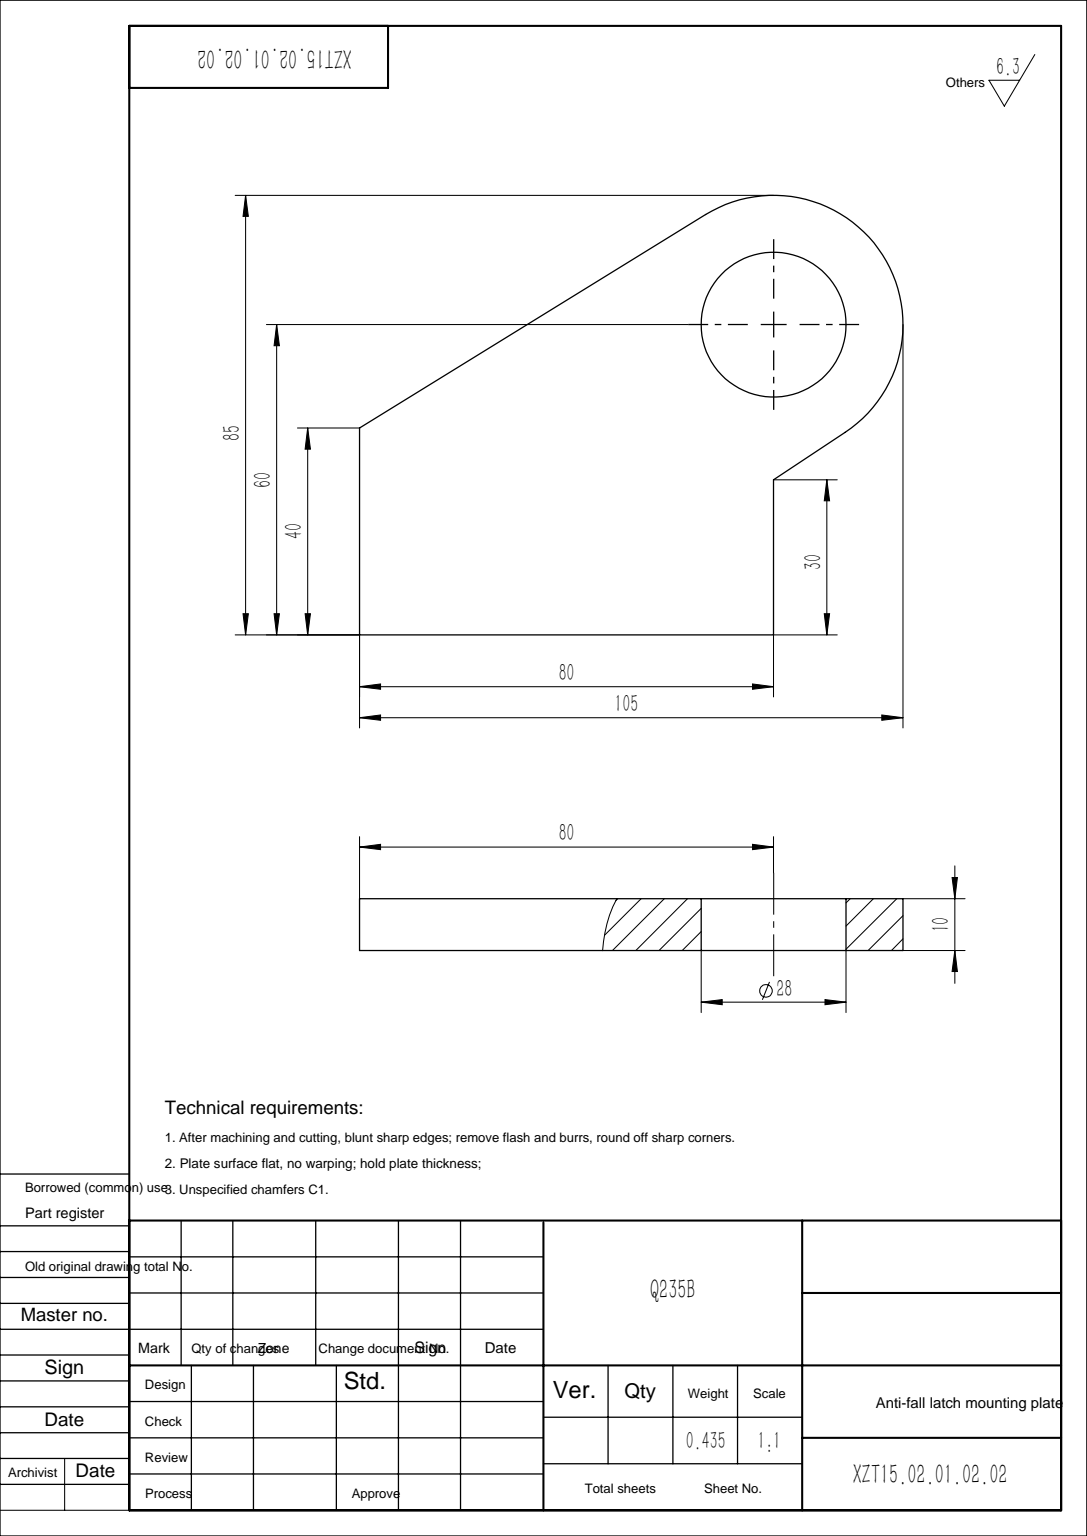
from build123d import *

# Parameters (mm, degrees)
SKETCH1_R           = 14
BOSS_EXTRUDE1_DEPTH = 5


with BuildPart() as part:
    # Sketch1 → Boss-Extrude1 (new, symmetric)
    with BuildSketch(Plane.XY):
        with BuildLine():
            Line((0, 0), (0, 40))
            Line((0, 40), (66.869031748, 81.273873008))
            ThreePointArc((66.869031748, 81.273873008), (101.056415799, 73.476919296), (93.81926996, 39.166666667))
            Line((93.81926996, 39.166666667), (80, 30))
            Line((80, 30), (80, 0))
            Line((80, 0), (0, 0))
        make_face()
        with Locations((80, 60)):
            Circle(SKETCH1_R, mode=Mode.SUBTRACT)
    extrude(amount=BOSS_EXTRUDE1_DEPTH, both=True)


solid = part.part
